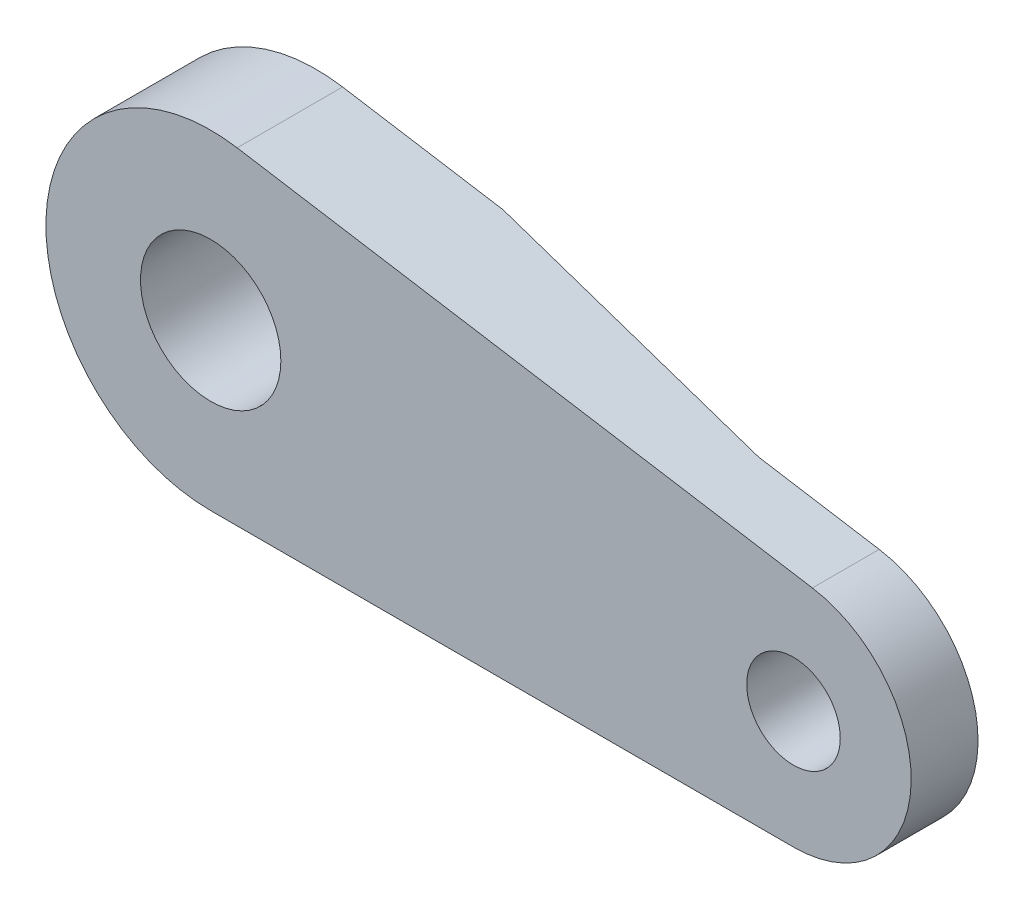
from build123d import *

# Parameters (mm, degrees)
SKETCH1_R               = 2
SKETCH1_R_2             = 3
BOSS_EXTRUDE1_DEPTH     = 6
CUT_EXTRUDE1_DEPTH      = 27.36555884
CUT_EXTRUDE1_DEPTH_BACK = 27.36555884


with BuildPart() as part:
    # Sketch1 → Boss-Extrude1 (new body)
    with BuildSketch(Plane.XY):
        with BuildLine():
            Line((-7.993562913, -0.787462727), (16.925257698, -0.787462727))
            ThreePointArc((16.925257698, -0.787462727), (21.941546469, 3.839929946), (17.733101807, 9.212537273))
            Line((17.733101807, 9.212537273), (-6.862581161, 13.212537273))
            ThreePointArc((-6.862581161, 13.212537273), (-15.016367191, 6.825553227), (-7.993562913, -0.787462727))
        make_face()
        with Locations((16.925257698, 4.245167879)):
            Circle(SKETCH1_R, mode=Mode.SUBTRACT)
        with Locations((-7.993562913, 6.258220121)):
            Circle(SKETCH1_R_2, mode=Mode.SUBTRACT)
    extrude(amount=BOSS_EXTRUDE1_DEPTH)

    # Sketch2 → Cut-Extrude1 (cut, two sides: drawn at the far end of the back side and taken through both)
    with BuildSketch(Plane(origin=(0, 0, 0), x_dir=(1, 0, 0), z_dir=(0, 1, 0)).offset(-CUT_EXTRUDE1_DEPTH_BACK)):
        Polygon((29.386629895, -3.141643917), (12.58106894, -3.141643917), (0, -1.491733663), (-17.019149761, -1.491733663), (-15.478750308, 10.25428202), (32.017830731, 8.260226372), align=None)
    extrude(amount=CUT_EXTRUDE1_DEPTH + CUT_EXTRUDE1_DEPTH_BACK, mode=Mode.SUBTRACT)


solid = part.part
